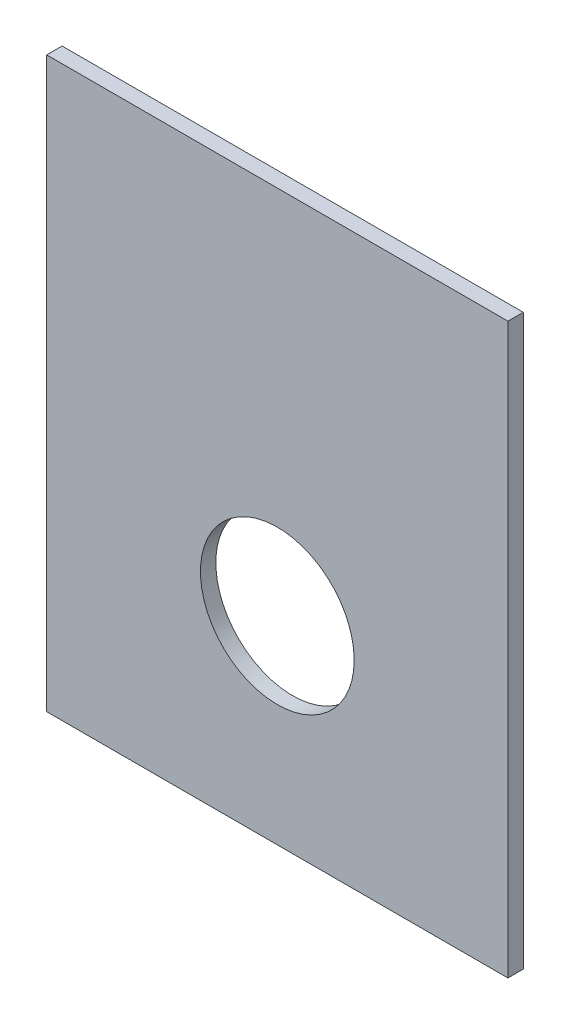
SolidWorks part; units mm, degrees
ref_plane "Front Plane" through (0, 0, 0) normal (0, 0, 1) x (1, 0, 0)
ref_plane "Top Plane" through (0, 0, 0) normal (0, 1, 0) x (1, 0, 0)
ref_plane "Right Plane" through (0, 0, 0) normal (1, 0, 0) x (0, 0, -1)
sketch "Sketch1" plane through (0, 0, 0) normal (0, 0, 1) x (1, 0, 0)
  line L1 (0, 0) -> (300, 0)
  line L2 (0, 0) -> (0, 370)
  line L3 (0, 370) -> (300, 370)
  line L4 (300, 0) -> (300, 370)
  circle A0 centre (150, 129) radius 50
  dimension "D5" = 100
  dimension "D1" = 300
  dimension "D2" = 370
  dimension "D3" = 129
  dimension "D4" = 150
extrude "Boss-Extrude1" add sketch "Sketch1" along normal blind 10
